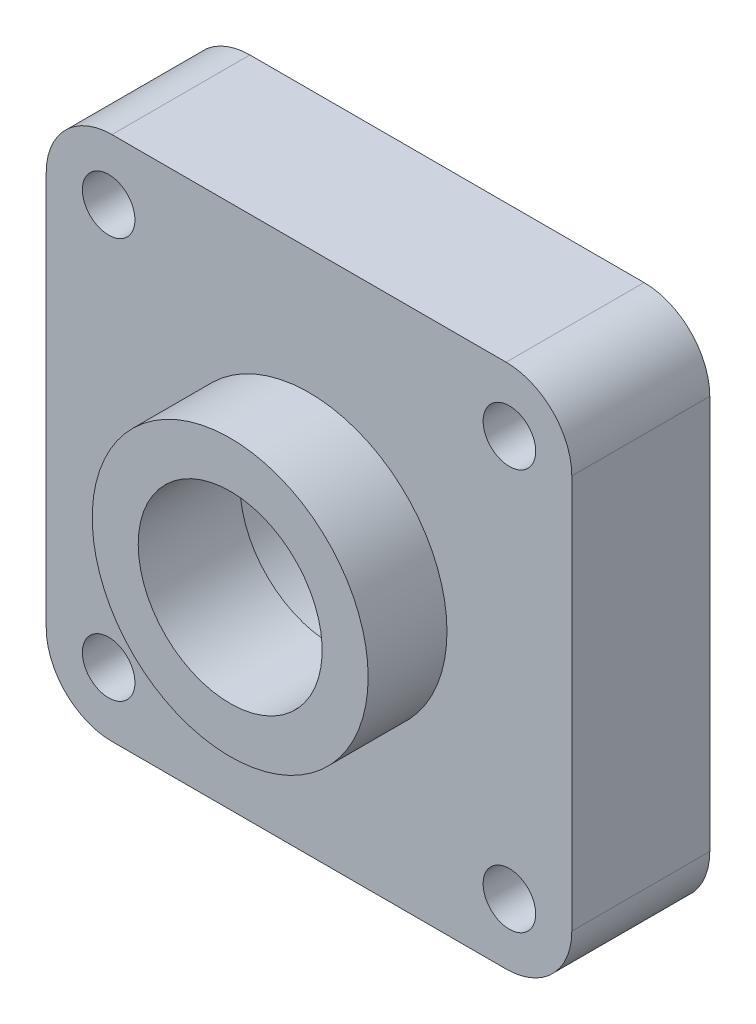
from build123d import *

# Parameters (mm, degrees)
SKETCH_1_W               = 80
SKETCH_1_H               = 80
EXTRUDE_1_DEPTH          = 21
SKETCH_2_R               = 21
EXTRUDE_2_DEPTH          = 12
FILLET_1_R               = 10
SKETCH_6_R               = 4
CUT_EXTRUDE_1_DEPTH      = 21
MIRROR_2_COPY_1_SKETCH_R = 4
MIRROR_2_COPY_1_DEPTH    = 21
FILLET_2_R               = 1
FILLET_3_R               = 1


with BuildPart() as part:
    # 草图1 → 凸台-拉伸1 (new body)
    with BuildSketch(Plane.XY):
        Rectangle(SKETCH_1_W, SKETCH_1_H)
    extrude(amount=EXTRUDE_1_DEPTH)

    # 草图2 → 凸台-拉伸2 (add)
    with BuildSketch(Plane.XY.offset(21)):
        Circle(SKETCH_2_R)
    extrude(amount=EXTRUDE_2_DEPTH)

    # 草图3 → 切除-旋转1 (revolve, cut)
    with BuildSketch(Plane(origin=(0, 0, 0), x_dir=(1, 0, 0), z_dir=(0, 1, 0)), mode=Mode.PRIVATE) as cut_revolve_1_sk:
        Polygon((30, 0), (30, -2.5), (22.5, -2.5), (22.5, -7.5), (17.5, -7.5), (17.5, -15.5), (20, -15.5), (20, -17.5), (14, -17.5), (14, -33), (0, -33), (0, 0), align=None)
    revolve(cut_revolve_1_sk.sketch.rotate(Axis((0, 0, 0), (0, 0, 1)), 180), axis=Axis((0, 0, 0), (0, 0, 1)), mode=Mode.SUBTRACT)

    # 圆角1
    fillet_1_edges = [part.edges().sort_by_distance(p)[0] for p in [
        (40, -40, 10.5),
        (-40, -40, 10.5),
        (-40, 40, 10.5),
        (40, 40, 10.5),
    ]]
    fillet(fillet_1_edges, radius=FILLET_1_R)

    # 草图6 → 切除-拉伸1 (cut)
    with BuildSketch(Plane.XY.offset(21)):
        with Locations((-30.5, 30.5)):
            Circle(SKETCH_6_R)
    cut_extrude_1 = extrude(amount=-CUT_EXTRUDE_1_DEPTH, mode=Mode.SUBTRACT)

    # 镜向1: 切除-拉伸1 across plane
    add(cut_extrude_1.mirror(Plane.ZX), mode=Mode.SUBTRACT)

    # 镜向2: 切除-拉伸1 across plane
    add(cut_extrude_1.mirror(Plane(origin=(0, 0, 0), x_dir=(0, 0, 1), z_dir=(1, 0, 0))), mode=Mode.SUBTRACT)

    # 镜向2 copy 1 sketch → 镜向2 copy 1 (cut)
    with BuildSketch(Plane(origin=(0, 0, 21), x_dir=(-1, 0, 0), z_dir=(0, 0, 1))):
        with Locations((-30.5, 30.5)):
            Circle(MIRROR_2_COPY_1_SKETCH_R)
    extrude(amount=-MIRROR_2_COPY_1_DEPTH, mode=Mode.SUBTRACT)

    # 圆角2
    fillet_2_edges = [part.edges().sort_by_distance(p)[0] for p in [
        (30, 0, 2.5),
    ]]
    fillet(fillet_2_edges, radius=FILLET_2_R)

    # 圆角3
    fillet_3_edges = [part.edges().sort_by_distance(p)[0] for p in [
        (20, 0, 17.5),
    ]]
    fillet(fillet_3_edges, radius=FILLET_3_R)


solid = part.part
